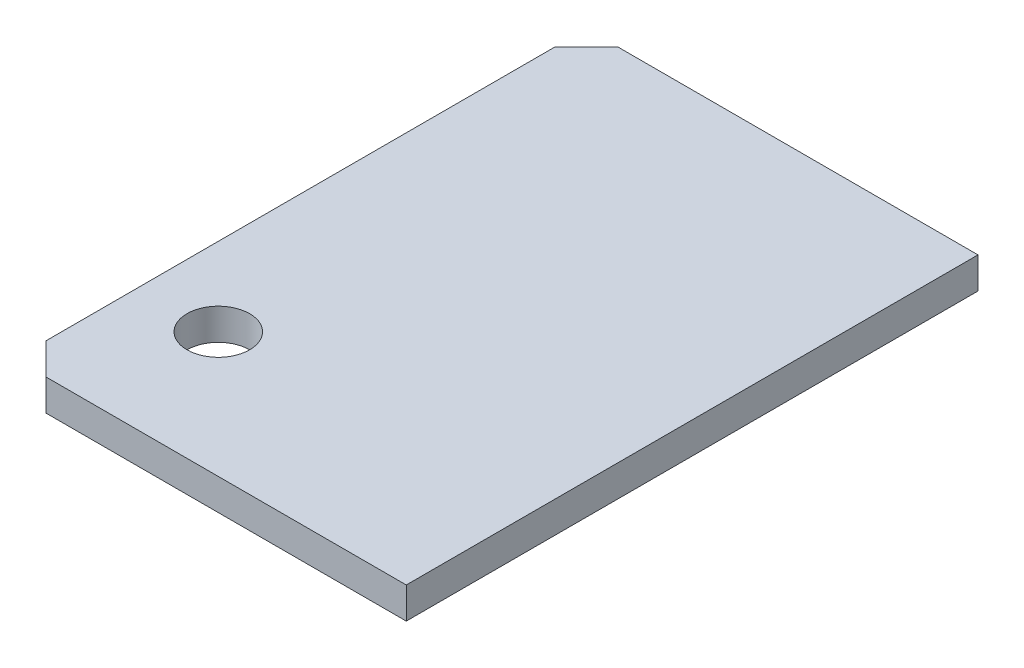
from build123d import *

# Parameters (mm, degrees)
SKETCH1_W               = 250
SKETCH1_H               = 20
BOSS_EXTRUDE1_DEPTH     = 365
CHAMFER1_SIZE           = 20
CUT_EXTRUDE1_DEPTH      = 443.860023032
CUT_EXTRUDE1_DEPTH_BACK = 443.860023032
SKETCH2_R               = 20
CHAMFER2_SIZE           = 20


with BuildPart() as part:
    # Sketch1 → Boss-Extrude1 (new body)
    with BuildSketch(Plane.XY):
        with Locations((-125, 10)):
            Rectangle(SKETCH1_W, SKETCH1_H)
    extrude(amount=BOSS_EXTRUDE1_DEPTH)

    # Chamfer1
    chamfer1_edges = [part.edges().sort_by_distance(p)[0] for p in [
        (-250, 10, 365),
    ]]
    chamfer(chamfer1_edges, length=CHAMFER1_SIZE)

    # Sketch2 → Cut-Extrude1 (cut, two sides: drawn at the far end of the back side and taken through both)
    with BuildSketch(Plane(origin=(0, 20, 0), x_dir=(1, 0, 0), z_dir=(0, 1, 0)).offset(-CUT_EXTRUDE1_DEPTH_BACK)):
        with Locations(Location((-200, -285, 0), (0, 0, 180))):
            Circle(SKETCH2_R)
    extrude(amount=CUT_EXTRUDE1_DEPTH + CUT_EXTRUDE1_DEPTH_BACK, mode=Mode.SUBTRACT)

    # Chamfer2
    chamfer2_edges = [part.edges().sort_by_distance(p)[0] for p in [
        (-250, 10, 0),
    ]]
    chamfer(chamfer2_edges, length=CHAMFER2_SIZE)


solid = part.part
